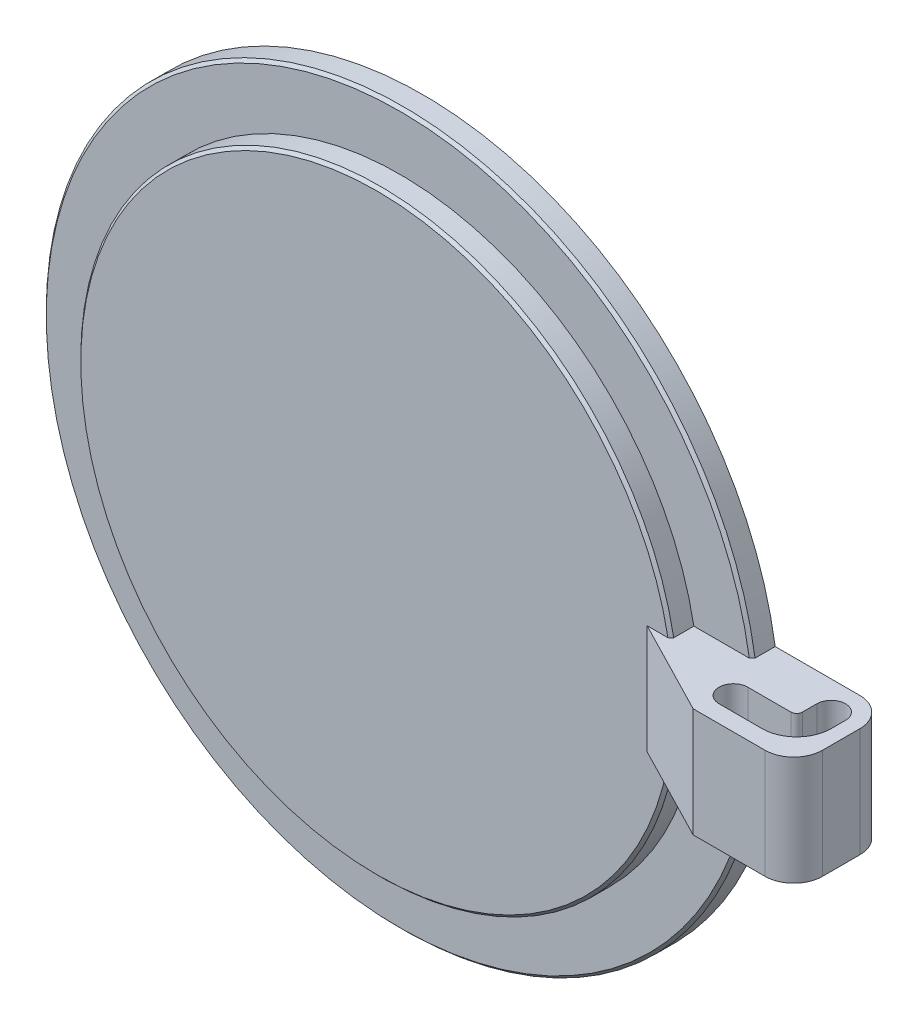
from build123d import *

# Parameters (mm, degrees)
SKETCH_1_R      = 62
EXTRUDE_1_DEPTH = 4
SKETCH_2_R      = 52
EXTRUDE_2_DEPTH = 4
EXTRUDE_3_DEPTH = 9.5
FILLET_1_R      = 5
CHAMFER_1_SIZE  = 0.5


with BuildPart() as part:
    # 草图1 → 凸台-拉伸1 (new body)
    with BuildSketch(Plane.XY):
        Circle(SKETCH_1_R)
    extrude(amount=EXTRUDE_1_DEPTH)

    # 草图2 → 凸台-拉伸2 (add)
    with BuildSketch(Plane.XY.offset(4)):
        Circle(SKETCH_2_R)
    extrude(amount=EXTRUDE_2_DEPTH)

    # 草图3 → 凸台-拉伸3 (add, symmetric)
    with BuildSketch(Plane(origin=(0, 0, 0), x_dir=(1, 0, 0), z_dir=(0, 1, 0))):
        with BuildLine():
            Line((81, 0), (81, -11.5))
            ThreePointArc((81, -11.5), (79.535533906, -15.035533906), (76, -16.5))
            Line((76, -16.5), (63.5, -16.5))
            Line((63.5, -16.5), (47, -8))
            Line((47, -8), (47, 0))
            Line((47, 0), (81, 0))
        make_face()
        with BuildLine():
            Line((73.5, -5), (73.5, -7.5))
            ThreePointArc((73.5, -7.5), (73.207106781, -8.207106781), (72.5, -8.5))
            Line((72.5, -8.5), (65, -8.5))
            ThreePointArc((65, -8.5), (62.5, -11), (65, -13.5))
            Line((65, -13.5), (72.5, -13.5))
            ThreePointArc((72.5, -13.5), (76.742640687, -11.742640687), (78.5, -7.5))
            Line((78.5, -7.5), (78.5, -5))
            ThreePointArc((78.5, -5), (76, -2.5), (73.5, -5))
        make_face(mode=Mode.SUBTRACT)
    extrude(amount=EXTRUDE_3_DEPTH, both=True)

    # 圆角1
    fillet_1_edges = [part.edges().sort_by_distance(p)[0] for p in [
        (81, 0, 0),
    ]]
    fillet(fillet_1_edges, radius=FILLET_1_R)

    # 倒角1
    chamfer_1_edges = [part.edges().sort_by_distance(p)[0] for p in [
        (-62, 0, 4),
        (-52, 0, 8),
    ]]
    chamfer(chamfer_1_edges, length=CHAMFER_1_SIZE)


solid = part.part
